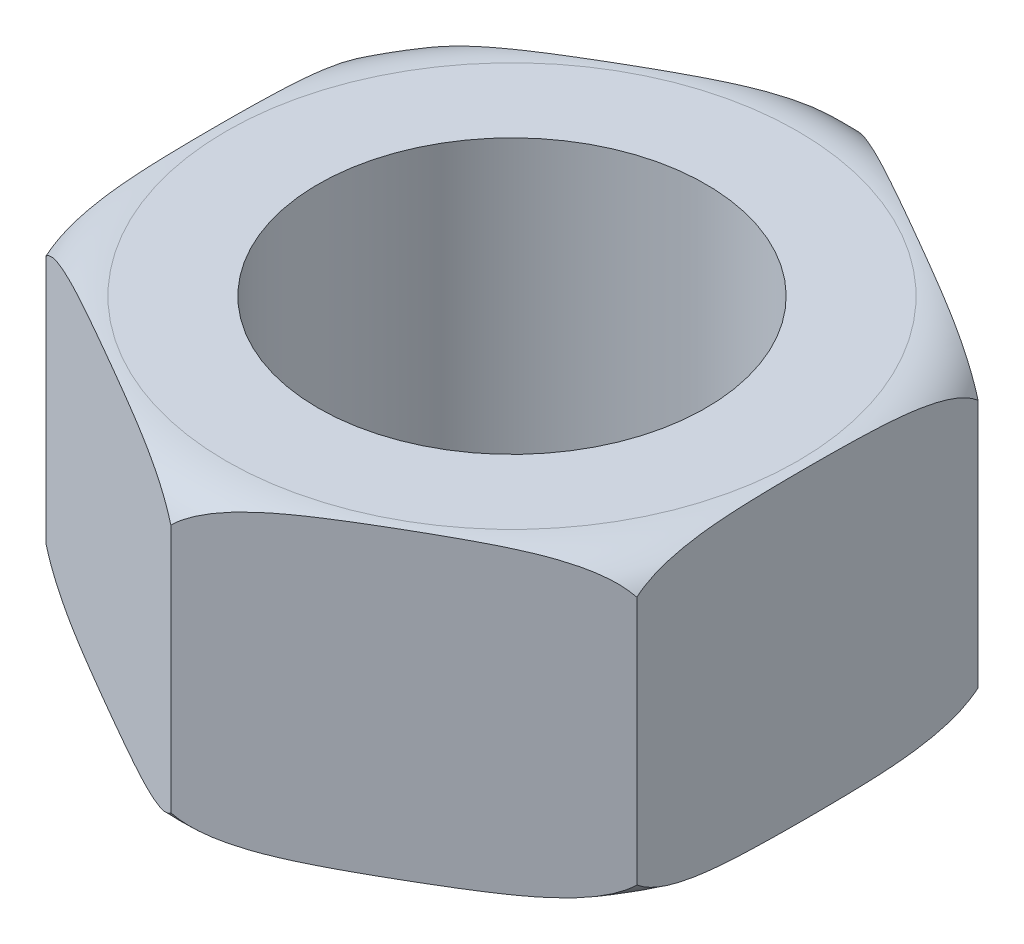
from build123d import *

# Parameters (mm, degrees)
SKETCH_1_R           = 21
BOSS_EXTRUDE_1_DEPTH = 16.5


with BuildPart() as part:
    # Sketch 1 → Boss-Extrude 1 (new, symmetric)
    with BuildSketch(Plane(origin=(0, 0, 0), x_dir=(1, 0, 0), z_dir=(0, 1, 0))):
        Polygon((0, 36.950417228), (-32, 18.475208614), (-32, -18.475208614), (0, -36.950417228), (32, -18.475208614), (32, 18.475208614), align=None)
        with Locations(Location((0, 0, 0), (0, 0, 270))):
            Circle(SKETCH_1_R, mode=Mode.SUBTRACT)
    extrude(amount=BOSS_EXTRUDE_1_DEPTH, both=True)

    # Sketch 2 → Cut-Revolve 1 (revolve, cut)
    with BuildSketch(Plane(origin=(0, 0, 0), x_dir=(0, 0, -1), z_dir=(1, 0, 0))):
        with BuildLine():
            Line((-30.950417228, 16.5), (-36.950417228, 16.5))
            Line((-36.950417228, 16.5), (-36.950417228, 13.5))
            add(Edge.make_bspline(
                [(-36.950417228, 13.5), (-35.688982599, 15.62896823), (-33.371774895, 16.5), (-30.950417228, 16.5)],
                knots=[0, 0, 0, 0, 1, 1, 1, 1], degree=3))
        make_face()
        with BuildLine():
            Line((-36.950417228, -16.5), (-36.950417228, -13.5))
            add(Edge.make_bspline(
                [(-36.950417228, -13.5), (-35.688982599, -15.62896823), (-33.371774895, -16.5), (-30.950417228, -16.5)],
                knots=[0, 0, 0, 0, 1, 1, 1, 1], degree=3))
            Line((-30.950417228, -16.5), (-36.950417228, -16.5))
        make_face()
    revolve(axis=Axis((0, 20.720193417, 0), (0, -1, 0)), mode=Mode.SUBTRACT)


solid = part.part
